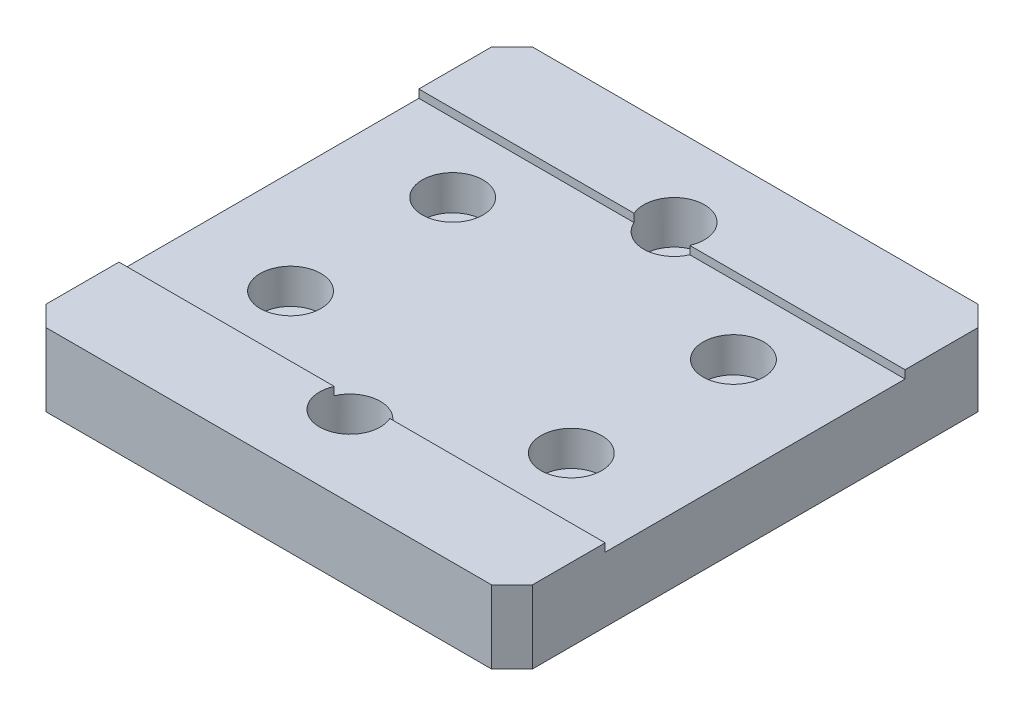
SolidWorks part; units mm, degrees
material "6061Al"
ref_plane "前视基准面" through (0, 0, 0) normal (0, 0, 1) x (1, 0, 0)
ref_plane "上视基准面" through (0, 0, 0) normal (0, 1, 0) x (1, 0, 0)
ref_plane "右视基准面" through (0, 0, 0) normal (1, 0, 0) x (0, 0, -1)
sketch "草图1" plane through (0, 0, 0) normal (0, 1, 0) x (1, 0, 0)
  line L1 (-60, -60) -> (60, -60)
  line L2 (-60, -60) -> (-60, 60)
  line L3 (-60, 60) -> (60, 60)
  line L4 (60, -60) -> (60, 60)
  line L5 (-60, -60) -> (60, 60) construction
  line L6 (-60, 60) -> (60, -60) construction
  point P0 (0, 0)
  dimension "D1" = 120
  dimension "D2" = 120
extrude "凸台-拉伸1" add sketch "草图1" along normal blind 18
hole_wizard "M8 六角凹头螺钉的柱形沉头孔3" positions "草图9" profile "草图10" counterbore size "M8" standard "ISO" end condition through all
sketch "草图9" plane through (0, 18, 0) normal (0, 1, 0) x (1, 0, 0)
  point P0 (0, 40)
  point P3 (-34.641, 20)
  point P6 (-34.641, -20)
  point P9 (0, -40)
  point P12 (34.641, -20)
  point P15 (34.641, 20)
sketch "草图10" plane through (0, 18, -40) normal (1, 0, 0) x (0, 0, 1)
  line L0 (0, 0) -> (0, 18)
  line L1 (0, 18) -> (4.5, 18)
  line L3 (4.5, 18) -> (4.5, 10.6)
  line L4 (4.5, 10.6) -> (7.5, 10.6)
  line L5 (7.5, 10.6) -> (7.5, 0)
  line L7 (7.5, 0) -> (0, 0)
  line L11 (0, -6.35) -> (0, 107.95) construction
  dimension "通孔孔直径" = 9
  dimension "通孔孔深度" = 18
  dimension "柱形沉头孔直径" = 15
  dimension "柱形沉头孔深度" = 10.6
sketch "草图11" plane through (0, 18, 0) normal (0, 1, 0) x (1, 0, 0)
  line L0 (60, -60) -> (60, 60) construction
  line L1 (-60, -37) -> (60, -37)
  line L2 (-60, -37) -> (-60, 37)
  line L3 (-60, 37) -> (60, 37)
  line L4 (60, -37) -> (60, 37)
  line L5 (-60, -37) -> (60, 37) construction
  line L6 (-60, 37) -> (60, -37) construction
  point P0 (0, 0)
  dimension "D1" = 74
extrude "切除-拉伸2" cut sketch "草图11" against normal blind 2
chamfer "倒角1" distance 5 angle 45 4 edges at (60, 9, 60) (-60, 9, 60) (-60, 9, -60) (60, 9, -60)
